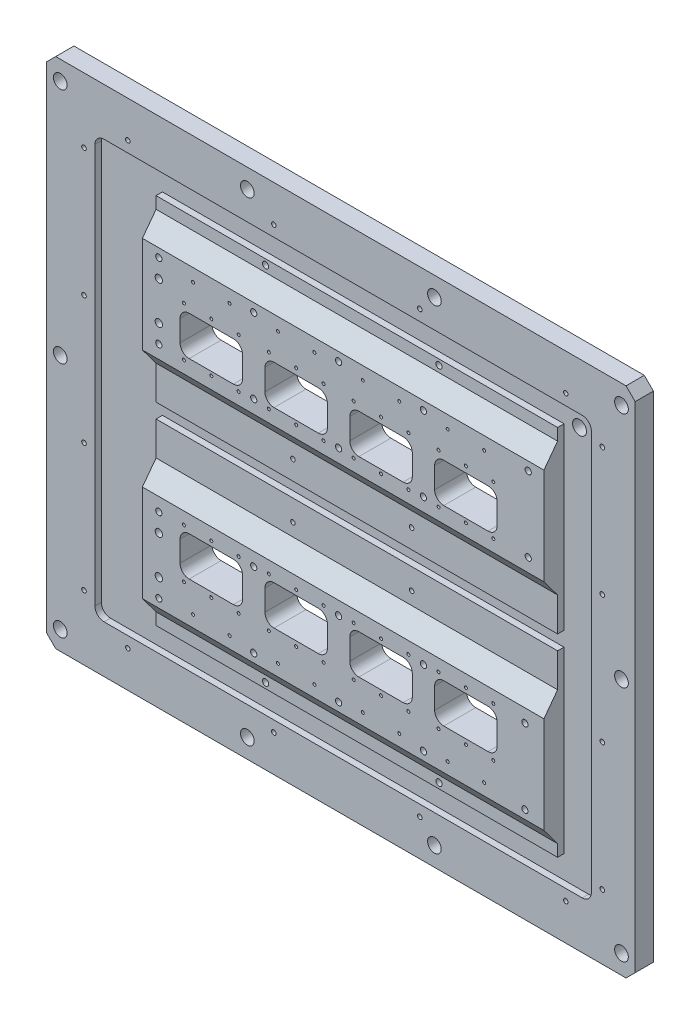
SolidWorks part; units mm, degrees
material "Q235-A"
ref_plane "Front Plane" through (0, 0, 0) normal (0, 0, 1) x (1, 0, 0)
ref_plane "Top Plane" through (0, 0, 0) normal (0, 1, 0) x (1, 0, 0)
ref_plane "Right Plane" through (0, 0, 0) normal (1, 0, 0) x (0, 0, -1)
sketch "Sketch1" plane through (0, 0, 0) normal (0, 0, 1) x (1, 0, 0)
  line L1 (-322.5, -281) -> (322.5, -281)
  line L2 (-322.5, -281) -> (-322.5, 281)
  line L3 (-322.5, 281) -> (322.5, 281)
  line L4 (322.5, -281) -> (322.5, 281)
  line L5 (-322.5, -281) -> (322.5, 281) construction
  line L6 (-322.5, 281) -> (322.5, -281) construction
  point P0 (0, 0)
  dimension "D1" = 562
  dimension "D2" = 645
extrude "Boss-Extrude1" add sketch "Sketch1" along normal blind 20
sketch "Sketch2" plane through (0, 0, 20) normal (0, 0, 1) x (1, 0, 0)
  line L0 (-322.5, 281) -> (-322.5, -281) construction
  line L1 (-269.5, 229) -> (274.5, 229)
  line L2 (-269.5, 229) -> (-269.5, -229)
  line L3 (-269.5, -229) -> (274.5, -229)
  line L4 (274.5, 229) -> (274.5, -229)
  line L5 (-322.5, -281) -> (322.5, -281) construction
  dimension "D1" = 544
  dimension "D2" = 53
  dimension "D3" = 52
  dimension "D4" = 458
extrude "Cut-Extrude1" cut sketch "Sketch2" against normal blind 7
chamfer "Chamfer1" distance 10 angle 45 4 edges at (322.5, -281, 10) (322.5, 281, 10) (-322.5, 281, 10) (-322.5, -281, 10)
ref_plane "Plane1" through (-202.5, 0, 0) normal (1, 0, 0) x (0, 0, -1)
sketch "Sketch3" plane through (-202.5, 0, 0) normal (1, 0, 0) x (0, 0, -1)
  line L0 (-13, 204) -> (-20, 204)
  line L1 (-13, -229) -> (-13, 229) construction
  line L2 (-20, -229) -> (-20, 229) construction
  line L5 (-35, 171) -> (-35, 65)
  line L8 (-20, 8) -> (-13, 8)
  line L9 (-13, 8) -> (-13, 204)
  line L10 (-20, 204) -> (-20, 191)
  line L11 (-20, -8) -> (-20, -45)
  line L14 (-13, -204) -> (-13, -8)
  line L15 (-20, -204) -> (-13, -204)
  line L17 (-13, -8) -> (-20, -8)
  line L18 (-35, -65) -> (-35, -171)
  line L20 (-13, -229) -> (-20, -229) construction
  line L21 (-20, -45) -> (-35, -65)
  line L22 (-20, -204) -> (-20, -191)
  line L23 (-20, -191) -> (-35, -171)
  line L24 (0, -281) -> (-20, -281) construction
  line L25 (0, -271) -> (0, 271) construction
  line L27 (-35, 65) -> (-20, 45)
  line L28 (-20, 45) -> (-20, 8)
  line L29 (-13, 229) -> (-20, 229) construction
  line L30 (-20, 191) -> (-35, 171)
  dimension "D2" = 35
  dimension "D3" = 106
  dimension "D4" = 35
  dimension "D5" = 25
  dimension "D6" = 7
  dimension "D7" = 16
  dimension "D8" = 25
  dimension "D9" = 20
  dimension "D10" = 146
  dimension "D11" = 106
  dimension "D12" = 273
  dimension "D13" = 146
  dimension "D14" = 20
  dimension "D15" = 236
  dimension "D16" = 90
extrude "Boss-Extrude2" add sketch "Sketch3" along normal blind 440
sketch "Sketch4" plane through (0, 0, 35) normal (0, 0, 1) x (1, 0, 0)
  line L0 (-312.5, -281) -> (312.5, -281) construction
  line L1 (-151.25, -83.74) -> (-102.75, -83.74)
  line L2 (-161.25, -93.74) -> (-161.25, -116.74)
  line L3 (-151.25, -126.74) -> (-102.75, -126.74)
  line L4 (-92.75, -93.74) -> (-92.75, -116.74)
  line L5 (-322.5, 271) -> (-322.5, -271) construction
  line L6 (-68.25, -93.74) -> (-68.25, -116.74)
  line L7 (-58.25, -83.74) -> (-9.75, -83.74)
  line L8 (0.25, -93.74) -> (0.25, -116.74)
  line L9 (-58.25, -126.74) -> (-9.75, -126.74)
  line L10 (24.75, -93.74) -> (24.75, -116.74)
  line L11 (34.75, -83.74) -> (83.25, -83.74)
  line L12 (93.25, -93.74) -> (93.25, -116.74)
  line L13 (34.75, -126.74) -> (83.25, -126.74)
  line L14 (117.75, -93.74) -> (117.75, -116.74)
  line L15 (127.75, -83.74) -> (176.25, -83.74)
  line L16 (186.25, -93.74) -> (186.25, -116.74)
  line L17 (127.75, -126.74) -> (176.25, -126.74)
  line L18 (-68.25, 115.5) -> (-68.25, 92.5)
  line L19 (-58.25, 125.5) -> (-9.75, 125.5)
  line L20 (0.25, 115.5) -> (0.25, 92.5)
  line L21 (-58.25, 82.5) -> (-9.75, 82.5)
  line L22 (24.75, 115.5) -> (24.75, 92.5)
  line L23 (34.75, 125.5) -> (83.25, 125.5)
  line L24 (93.25, 115.5) -> (93.25, 92.5)
  line L25 (34.75, 82.5) -> (83.25, 82.5)
  line L26 (117.75, 115.5) -> (117.75, 92.5)
  line L27 (127.75, 125.5) -> (176.25, 125.5)
  line L28 (186.25, 115.5) -> (186.25, 92.5)
  line L29 (127.75, 82.5) -> (176.25, 82.5)
  line L30 (-161.25, 115.5) -> (-161.25, 92.5)
  line L31 (-151.25, 125.5) -> (-102.75, 125.5)
  line L32 (-92.75, 115.5) -> (-92.75, 92.5)
  line L33 (-151.25, 82.5) -> (-102.75, 82.5)
  arc A0 (-102.75, -83.74) -> (-92.75, -93.74) centre (-102.75, -93.74) cw
  arc A1 (-92.75, -116.74) -> (-102.75, -126.74) centre (-102.75, -116.74) cw
  arc A2 (-151.25, -126.74) -> (-161.25, -116.74) centre (-151.25, -116.74) cw
  arc A3 (-161.25, -93.74) -> (-151.25, -83.74) centre (-151.25, -93.74) cw
  arc A4 (-68.25, -93.74) -> (-58.25, -83.74) centre (-58.25, -93.74) cw
  arc A5 (-58.25, -126.74) -> (-68.25, -116.74) centre (-58.25, -116.74) cw
  arc A6 (-9.75, -83.74) -> (0.25, -93.74) centre (-9.75, -93.74) cw
  arc A7 (0.25, -116.74) -> (-9.75, -126.74) centre (-9.75, -116.74) cw
  arc A8 (24.75, -93.74) -> (34.75, -83.74) centre (34.75, -93.74) cw
  arc A9 (34.75, -126.74) -> (24.75, -116.74) centre (34.75, -116.74) cw
  arc A10 (83.25, -83.74) -> (93.25, -93.74) centre (83.25, -93.74) cw
  arc A11 (93.25, -116.74) -> (83.25, -126.74) centre (83.25, -116.74) cw
  arc A12 (117.75, -93.74) -> (127.75, -83.74) centre (127.75, -93.74) cw
  arc A13 (127.75, -126.74) -> (117.75, -116.74) centre (127.75, -116.74) cw
  arc A14 (176.25, -83.74) -> (186.25, -93.74) centre (176.25, -93.74) cw
  arc A15 (186.25, -116.74) -> (176.25, -126.74) centre (176.25, -116.74) cw
  arc A16 (-68.25, 115.5) -> (-58.25, 125.5) centre (-58.25, 115.5) cw
  arc A17 (-58.25, 82.5) -> (-68.25, 92.5) centre (-58.25, 92.5) cw
  arc A18 (-9.75, 125.5) -> (0.25, 115.5) centre (-9.75, 115.5) cw
  arc A19 (0.25, 92.5) -> (-9.75, 82.5) centre (-9.75, 92.5) cw
  arc A20 (24.75, 115.5) -> (34.75, 125.5) centre (34.75, 115.5) cw
  arc A21 (34.75, 82.5) -> (24.75, 92.5) centre (34.75, 92.5) cw
  arc A22 (83.25, 125.5) -> (93.25, 115.5) centre (83.25, 115.5) cw
  arc A23 (93.25, 92.5) -> (83.25, 82.5) centre (83.25, 92.5) cw
  arc A24 (117.75, 115.5) -> (127.75, 125.5) centre (127.75, 115.5) cw
  arc A25 (127.75, 82.5) -> (117.75, 92.5) centre (127.75, 92.5) cw
  arc A26 (176.25, 125.5) -> (186.25, 115.5) centre (176.25, 115.5) cw
  arc A27 (186.25, 92.5) -> (176.25, 82.5) centre (176.25, 92.5) cw
  arc A28 (-161.25, 115.5) -> (-151.25, 125.5) centre (-151.25, 115.5) cw
  arc A29 (-151.25, 82.5) -> (-161.25, 92.5) centre (-151.25, 92.5) cw
  arc A30 (-102.75, 125.5) -> (-92.75, 115.5) centre (-102.75, 115.5) cw
  arc A31 (-92.75, 92.5) -> (-102.75, 82.5) centre (-102.75, 92.5) cw
  point P10 (-92.75, -83.74)
  point P15 (-161.25, -126.74)
  point P18 (-161.25, -83.74)
  dimension "D5" = 10
  dimension "D1" = 68.5
  dimension "D2" = 43
  dimension "D3" = 154.26
  dimension "D4" = 161.25
  dimension "D6" = 4
  dimension "D7" = 2
extrude "Cut-Extrude2" cut sketch "Sketch4" against normal blind 440
sketch "Sketch5" plane through (0, 0, 20) normal (0, 0, 1) x (1, 0, 0)
  line L0 (-312.5, -281) -> (312.5, -281) construction
  line L1 (-322.5, 271) -> (-322.5, -271) construction
  circle A0 centre (-307.5, -260) radius 11.6351
  circle A1 centre (-102.5, -260) radius 11.6351
  circle A2 centre (102.5, -260) radius 11.6351
  circle A3 centre (307.5, -260) radius 11.6351
  circle A4 centre (-102.5, 0) radius 11.6351
  circle A5 centre (102.5, 0) radius 11.6351
  circle A6 centre (307.5, 0) radius 11.6351
  circle A7 centre (-102.5, 260) radius 11.6351
  circle A8 centre (102.5, 260) radius 11.6351
  circle A9 centre (307.5, 260) radius 11.6351
  circle A10 centre (-307.5, 0) radius 11.6351
  circle A11 centre (-307.5, 260) radius 11.6351
  dimension "D1" = 21
  dimension "D2" = 15
  dimension "D3" = 4
  dimension "D4" = 3
hole_wizard "Hole1" positions "Sketch6" profile "Sketch7" legacy end condition through all
sketch "Sketch6" plane through (0, 0, 20) normal (0, 0, 1) x (1, 0, 0)
  point P0 (-307.5, 260)
  point P3 (-102.5, 260)
  point P6 (102.5, 260)
  point P9 (307.5, 260)
  point P12 (307.5, 0)
  point P15 (307.5, -260)
  point P18 (102.5, -260)
  point P21 (-102.5, -260)
  point P24 (-307.5, -260)
  point P27 (-307.5, 0)
sketch "Sketch7" plane through (-307.5, 260, 20) normal (1, 0, 0) x (0, -1, 0)
  line L0 (0, 0) -> (0, 20)
  line L1 (0, 20) -> (4.2, 20)
  line L2 (4.2, 20) -> (4.2, 11)
  line L3 (4.2, 11) -> (7.5, 11)
  line L4 (7.5, 11) -> (7.5, 0)
  line L5 (7.5, 0) -> (0, 0)
  line L6 (0, 110) -> (0, -10) construction
  dimension "直径" = 8.4
  dimension "深度" = 20
  dimension "柱坑直径" = 15
  dimension "柱坑深度" = 11
fillet "Fillet1" radius 10 4 edges at (-269.5, -229, 16.5) (274.5, -229, 16.5) (274.5, 229, 16.5) (-269.5, 229, 16.5)
sketch "Sketch8" plane through (0, 0, 20) normal (0, 0, 1) x (1, 0, 0)
  line L0 (-312.5, -281) -> (312.5, -281) construction
  line L1 (-322.5, 271) -> (-322.5, -271) construction
  circle A0 centre (-281.5, -210) radius 7.3177
  circle A1 centre (286.5, -210) radius 7.3177
  circle A2 centre (286.5, -70) radius 7.3177
  circle A3 centre (286.5, 70) radius 7.3177
  circle A4 centre (286.5, 210) radius 7.3177
  circle A5 centre (-281.5, -70) radius 7.3177
  circle A6 centre (-281.5, 70) radius 7.3177
  circle A7 centre (-281.5, 210) radius 7.3177
  circle A8 centre (-233.5, -241) radius 6.7741
  circle A9 centre (-73.5, -241) radius 6.7741
  circle A10 centre (86.5, -241) radius 6.7741
  circle A11 centre (246.5, -241) radius 6.7741
  circle A12 centre (-73.5, 241) radius 6.7741
  circle A13 centre (86.5, 241) radius 6.7741
  circle A14 centre (246.5, 241) radius 6.7741
  circle A15 centre (-233.5, 241) radius 6.7741
  dimension "D1" = 71
  dimension "D6" = 40
  dimension "D2" = 41
  dimension "D5" = 89
  dimension "D3" = 2
  dimension "D4" = 4
  dimension "D7" = 4
  dimension "D8" = 2
hole_wizard "M6 Tapped Hole1" positions "Sketch9" profile "Sketch10" tap size "M6" standard "GB"
sketch "Sketch9" plane through (0, 0, 20) normal (0, 0, 1) x (1, 0, 0)
  point P0 (-281.5, -210)
  point P3 (-233.5, -241)
  point P6 (-73.5, -241)
  point P9 (86.5, -241)
  point P12 (246.5, -241)
  point P23 (286.5, 70)
  point P26 (286.5, 210)
  point P29 (246.5, 241)
  point P32 (86.5, 241)
  point P35 (-73.5, 241)
  point P38 (-233.5, 241)
  point P41 (-281.5, 210)
  point P44 (-281.5, 70)
  point P50 (286.5, -210)
  point P57 (286.5, -70)
  point P61 (-281.5, -70)
sketch "Sketch10" plane through (-281.5, -210, 20) normal (1, 0, 0) x (0, -1, 0)
  line L0 (0, 0) -> (0, 11.5022)
  line L1 (0, 11.5022) -> (2.5, 10)
  line L2 (2.5, 10) -> (2.5, 0)
  line L5 (2.5, 0) -> (0, 0)
  line L10 (0, 11.5022) -> (-2.5, 10) construction
  line L11 (0, -6.35) -> (0, 107.95) construction
  dimension "螺纹孔钻头直径" = 5
  dimension "螺纹孔钻头深度" = 10
  dimension "导头角度" = 118
cosmetic thread "Cosmetic Thread1" parameters "D1"=10, "D2"=6
cosmetic thread "Cosmetic Thread2" parameters "D1"=10, "D2"=6
cosmetic thread "Cosmetic Thread3" parameters "D1"=10, "D2"=6
cosmetic thread "Cosmetic Thread4" parameters "D1"=10, "D2"=6
cosmetic thread "Cosmetic Thread5" parameters "D1"=10, "D2"=6
cosmetic thread "Cosmetic Thread6" parameters "D1"=10, "D2"=6
cosmetic thread "Cosmetic Thread7" parameters "D1"=10, "D2"=6
cosmetic thread "Cosmetic Thread8" parameters "D1"=10, "D2"=6
cosmetic thread "Cosmetic Thread9" parameters "D1"=10, "D2"=6
cosmetic thread "Cosmetic Thread10" parameters "D1"=10, "D2"=6
cosmetic thread "Cosmetic Thread11" parameters "D1"=10, "D2"=6
cosmetic thread "Cosmetic Thread12" parameters "D1"=10, "D2"=6
cosmetic thread "Cosmetic Thread13" parameters "D1"=10, "D2"=6
cosmetic thread "Cosmetic Thread14" parameters "D1"=10, "D2"=6
cosmetic thread "Cosmetic Thread15" parameters "D1"=10, "D2"=6
cosmetic thread "Cosmetic Thread16" parameters "D1"=10, "D2"=6
sketch "Sketch11" plane through (0, 0, 13) normal (0, 0, 1) x (1, 0, 0)
  line L0 (274.5, -219) -> (274.5, 219) construction
  line L1 (312.5, 281) -> (-312.5, 281) construction
  circle A0 centre (254.5, 209) radius 8.0509
  dimension "D1" = 20
  dimension "D2" = 72
hole_wizard "G3/8 Tapped Hole1" positions "Sketch12" profile "Sketch13" tap size "G3/8" standard "GB" end condition through all
sketch "Sketch12" plane through (0, 0, 13) normal (0, 0, 1) x (1, 0, 0)
  point P0 (254.5, 209)
sketch "Sketch13" plane through (254.5, 209, 13) normal (1, 0, 0) x (0, -1, 0)
  line L0 (0, 0) -> (0, 13)
  line L1 (0, 13) -> (7.625, 13)
  line L2 (7.625, 13) -> (7.625, 0)
  line L5 (7.625, 0) -> (0, 0)
  line L11 (0, -6.35) -> (0, 107.95) construction
  dimension "通孔螺纹孔钻头直径" = 15.25
  dimension "通孔螺纹孔钻头深度" = 13
cosmetic thread "Cosmetic Thread17" parameters "D2"=16.662
sketch "Sketch14" plane through (0, 0, 0) normal (0, 0, -1) x (-1, 0, 0)
  line L0 (312.5, -281) -> (-312.5, -281) construction
  line L1 (322.5, 271) -> (322.5, -271) construction
  circle A0 centre (187.5, -166) radius 10.1136
  circle A1 centre (87.5, -166) radius 10.1136
  circle A2 centre (-12.5, -166) radius 10.1136
  circle A3 centre (-112.5, -166) radius 10.1136
  circle A4 centre (-212.5, -166) radius 10.1136
  circle A5 centre (87.5, -24) radius 10.1136
  circle A6 centre (-12.5, -24) radius 10.1136
  circle A7 centre (-112.5, -24) radius 10.1136
  circle A8 centre (-212.5, -24) radius 10.1136
  circle A9 centre (187.5, -24) radius 10.1136
  circle A10 centre (187.5, 28) radius 10.1136
  circle A11 centre (87.5, 28) radius 10.1136
  circle A12 centre (187.5, 170) radius 10.1136
  circle A13 centre (87.5, 170) radius 10.1136
  circle A14 centre (-12.5, 170) radius 10.1136
  circle A15 centre (-112.5, 170) radius 10.1136
  circle A16 centre (-212.5, 170) radius 10.1136
  circle A17 centre (-212.5, 28) radius 10.1136
  circle A18 centre (-112.5, 28) radius 10.1136
  circle A19 centre (-12.5, 28) radius 10.1136
  dimension "D1" = 115
  dimension "D2" = 135
  dimension "D3" = 5
  dimension "D4" = 2
  dimension "D5" = 2
hole_wizard "M8 Tapped Hole1" positions "Sketch15" profile "Sketch16" tap size "M8" standard "GB"
sketch "Sketch15" plane through (0, 0, 0) normal (0, 0, -1) x (-1, 0, 0)
  point P0 (-212.5, 170)
  point P3 (-112.5, 170)
  point P6 (-12.5, 170)
  point P9 (87.5, 170)
  point P12 (187.5, 170)
  point P15 (187.5, 28)
  point P18 (87.5, 28)
  point P21 (-12.5, 28)
  point P24 (-112.5, 28)
  point P27 (-212.5, 28)
  point P30 (-212.5, -24)
  point P33 (-212.5, -166)
  point P36 (-112.5, -166)
  point P39 (-112.5, -24)
  point P42 (-12.5, -24)
  point P45 (87.5, -24)
  point P48 (187.5, -24)
  point P51 (187.5, -166)
  point P54 (87.5, -166)
  point P57 (-12.5, -166)
sketch "Sketch16" plane through (212.5, 170, 0) normal (1, 0, 0) x (0, 1, 0)
  line L0 (0, 0) -> (0, 18.0429)
  line L1 (0, 18.0429) -> (3.4, 16)
  line L2 (3.4, 16) -> (3.4, 0)
  line L5 (3.4, 0) -> (0, 0)
  line L10 (0, 18.0429) -> (-3.4, 16) construction
  line L11 (0, -6.35) -> (0, 107.95) construction
  dimension "螺纹孔钻头直径" = 6.8
  dimension "螺纹孔钻头深度" = 16
  dimension "导头角度" = 118
cosmetic thread "Cosmetic Thread18" parameters "D1"=16, "D2"=8
cosmetic thread "Cosmetic Thread19" parameters "D1"=16, "D2"=8
cosmetic thread "Cosmetic Thread20" parameters "D1"=16, "D2"=8
cosmetic thread "Cosmetic Thread21" parameters "D1"=16, "D2"=8
cosmetic thread "Cosmetic Thread22" parameters "D1"=16, "D2"=8
cosmetic thread "Cosmetic Thread23" parameters "D1"=16, "D2"=8
cosmetic thread "Cosmetic Thread24" parameters "D1"=16, "D2"=8
cosmetic thread "Cosmetic Thread25" parameters "D1"=16, "D2"=8
cosmetic thread "Cosmetic Thread26" parameters "D1"=16, "D2"=8
cosmetic thread "Cosmetic Thread27" parameters "D1"=16, "D2"=8
cosmetic thread "Cosmetic Thread28" parameters "D1"=16, "D2"=8
cosmetic thread "Cosmetic Thread29" parameters "D1"=16, "D2"=8
cosmetic thread "Cosmetic Thread30" parameters "D1"=16, "D2"=8
cosmetic thread "Cosmetic Thread31" parameters "D1"=16, "D2"=8
cosmetic thread "Cosmetic Thread32" parameters "D1"=16, "D2"=8
cosmetic thread "Cosmetic Thread33" parameters "D1"=16, "D2"=8
cosmetic thread "Cosmetic Thread34" parameters "D1"=16, "D2"=8
cosmetic thread "Cosmetic Thread35" parameters "D1"=16, "D2"=8
cosmetic thread "Cosmetic Thread36" parameters "D1"=16, "D2"=8
cosmetic thread "Cosmetic Thread37" parameters "D1"=16, "D2"=8
sketch "Sketch17" plane through (0, 0, 35) normal (0, 0, 1) x (1, 0, 0)
  line L0 (-322.5, 271) -> (-322.5, -271) construction
  line L1 (-312.5, -281) -> (312.5, -281) construction
  line L4 (-322.5, 0) -> (322.5, 0) construction
  line L5 (322.5, -271) -> (322.5, 271) construction
  line L6 (-184.5, 161.6) -> (-184.5, -161.6) construction
  circle A0 centre (-184.5, -161.6) radius 8.2899
  circle A1 centre (-80.5, -161.6) radius 8.2899
  circle A2 centre (-80.5, -79.6) radius 8.2899
  circle A3 centre (-184.5, -79.6) radius 8.2899
  circle A4 centre (12.5, -161.6) radius 8.2899
  circle A5 centre (12.5, -79.6) radius 8.2899
  circle A6 centre (105.5, -161.6) radius 8.2899
  circle A7 centre (105.5, -79.6) radius 8.2899
  circle A8 centre (216.7, -161.6) radius 8.2899
  circle A9 centre (216.7, -79.6) radius 8.2899
  circle A10 centre (220.3, 79.6) radius 8.2899
  circle A11 centre (220.3, 161.6) radius 8.2899
  circle A12 centre (105.5, 79.6) radius 8.2899
  circle A13 centre (105.5, 161.6) radius 8.2899
  circle A14 centre (12.5, 79.6) radius 8.2899
  circle A15 centre (12.5, 161.6) radius 8.2899
  circle A16 centre (-184.5, 79.6) radius 8.2899
  circle A17 centre (-80.5, 79.6) radius 8.2899
  circle A18 centre (-80.5, 161.6) radius 8.2899
  circle A19 centre (-184.5, 161.6) radius 8.2899
  circle A20 centre (-184.5, 141.6) radius 4.5108
  circle A21 centre (-184.5, 99.6) radius 4.7491
  circle A22 centre (-184.5, -99.6) radius 4.5108
  circle A23 centre (-184.5, -141.6) radius 4.7491
  dimension "D1" = 138
  dimension "D2" = 119.4
  dimension "D8" = 20
  dimension "D9" = 42
  dimension "D10" = 114.8
  dimension "D11" = 114.8
  dimension "D3" = 2
  dimension "D4" = 2
  dimension "D5" = 2
  dimension "D6" = 2
  dimension "D7" = 2
hole_wizard "Hole2" positions "Sketch18" profile "Sketch19" legacy
sketch "Sketch18" plane through (0, 0, 35) normal (0, 0, 1) x (1, 0, 0)
  point P0 (-184.5, 141.6)
  point P3 (-184.5, 99.6)
  point P6 (-184.5, -99.6)
  point P9 (-184.5, -141.6)
sketch "Sketch19" plane through (-184.5, 141.6, 35) normal (1, 0, 0) x (0, -1, 0)
  line L0 (0, 0) -> (0, 8.5)
  line L1 (0, 8.5) -> (4, 8.5)
  line L2 (4, 8.5) -> (4, 0)
  line L3 (4, 0) -> (0, 0)
  line L4 (0, 110) -> (0, -10) construction
  dimension "直径" = 8
  dimension "深度" = 8.5
hole_wizard "M8 Tapped Hole2" positions "Sketch20" profile "Sketch21" tap size "M8" standard "GB"
sketch "Sketch20" plane through (0, 0, 35) normal (0, 0, 1) x (1, 0, 0)
  point P0 (-184.5, 161.6)
  point P3 (-80.5, 161.6)
  point P6 (12.5, 161.6)
  point P9 (105.5, 161.6)
  point P12 (220.3, 161.6)
  point P15 (220.3, 79.6)
  point P18 (105.5, 79.6)
  point P21 (12.5, 79.6)
  point P24 (-80.5, 79.6)
  point P27 (-184.5, 79.6)
  point P30 (-184.5, -79.6)
  point P33 (-184.5, -161.6)
  point P36 (-80.5, -161.6)
  point P39 (-80.5, -79.6)
  point P42 (12.5, -79.6)
  point P45 (12.5, -161.6)
  point P48 (105.5, -161.6)
  point P51 (105.5, -79.6)
  point P54 (216.7, -79.6)
  point P57 (216.7, -161.6)
sketch "Sketch21" plane through (-184.5, 161.6, 35) normal (1, 0, 0) x (0, -1, 0)
  line L0 (0, 0) -> (0, 18.0429)
  line L1 (0, 18.0429) -> (3.4, 16)
  line L2 (3.4, 16) -> (3.4, 0)
  line L5 (3.4, 0) -> (0, 0)
  line L10 (0, 18.0429) -> (-3.4, 16) construction
  line L11 (0, -6.35) -> (0, 107.95) construction
  dimension "螺纹孔钻头直径" = 6.8
  dimension "螺纹孔钻头深度" = 16
  dimension "导头角度" = 118
cosmetic thread "Cosmetic Thread38" parameters "D1"=16, "D2"=8
cosmetic thread "Cosmetic Thread39" parameters "D1"=16, "D2"=8
cosmetic thread "Cosmetic Thread40" parameters "D1"=16, "D2"=8
cosmetic thread "Cosmetic Thread41" parameters "D1"=16, "D2"=8
cosmetic thread "Cosmetic Thread42" parameters "D1"=16, "D2"=8
cosmetic thread "Cosmetic Thread43" parameters "D1"=16, "D2"=8
cosmetic thread "Cosmetic Thread44" parameters "D1"=16, "D2"=8
cosmetic thread "Cosmetic Thread45" parameters "D1"=16, "D2"=8
cosmetic thread "Cosmetic Thread46" parameters "D1"=16, "D2"=8
cosmetic thread "Cosmetic Thread47" parameters "D1"=16, "D2"=8
cosmetic thread "Cosmetic Thread48" parameters "D1"=16, "D2"=8
cosmetic thread "Cosmetic Thread49" parameters "D1"=16, "D2"=8
cosmetic thread "Cosmetic Thread50" parameters "D1"=16, "D2"=8
cosmetic thread "Cosmetic Thread51" parameters "D1"=16, "D2"=8
cosmetic thread "Cosmetic Thread52" parameters "D1"=16, "D2"=8
cosmetic thread "Cosmetic Thread53" parameters "D1"=16, "D2"=8
cosmetic thread "Cosmetic Thread54" parameters "D1"=16, "D2"=8
cosmetic thread "Cosmetic Thread55" parameters "D1"=16, "D2"=8
cosmetic thread "Cosmetic Thread56" parameters "D1"=16, "D2"=8
cosmetic thread "Cosmetic Thread57" parameters "D1"=16, "D2"=8
sketch "Sketch22" plane through (0, 0, 35) normal (0, 0, 1) x (1, 0, 0)
  line L0 (-322.5, 271) -> (-322.5, -271) construction
  line L1 (-312.5, -281) -> (312.5, -281) construction
  circle A0 centre (-147, 157) radius 5.3737
  circle A1 centre (-107, 157) radius 5.3737
  circle A2 centre (-107, -158.24) radius 5.3737
  circle A3 centre (-147, -158.24) radius 5.3737
  circle A4 centre (-54, -158.24) radius 5.3737
  circle A5 centre (-14, -158.24) radius 5.3737
  circle A6 centre (-54, 157) radius 5.3737
  circle A7 centre (-14, 157) radius 5.3737
  circle A8 centre (39, -158.24) radius 5.3737
  circle A9 centre (79, -158.24) radius 5.3737
  circle A10 centre (39, 157) radius 5.3737
  circle A11 centre (79, 157) radius 5.3737
  circle A12 centre (132, -158.24) radius 5.3737
  circle A13 centre (172, -158.24) radius 5.3737
  circle A14 centre (132, 157) radius 5.3737
  circle A15 centre (172, 157) radius 5.3737
  dimension "D2" = 438
  dimension "D1" = 175.5
  dimension "D3" = 2
  dimension "D4" = 2
  dimension "D5" = 4
hole_wizard "M4 Tapped Hole1" positions "Sketch23" profile "Sketch24" tap size "M4" standard "GB"
sketch "Sketch23" plane through (0, 0, 35) normal (0, 0, 1) x (1, 0, 0)
  point P0 (-147, 157)
  point P3 (-107, 157)
  point P6 (-54, 157)
  point P9 (-14, 157)
  point P12 (39, 157)
  point P15 (79, 157)
  point P18 (132, 157)
  point P21 (172, 157)
  point P24 (-147, -158.24)
  point P27 (-107, -158.24)
  point P30 (-54, -158.24)
  point P33 (-14, -158.24)
  point P36 (39, -158.24)
  point P39 (79, -158.24)
  point P42 (132, -158.24)
  point P45 (172, -158.24)
sketch "Sketch24" plane through (-147, 157, 35) normal (1, 0, 0) x (0, -1, 0)
  line L0 (0, 0) -> (0, 8.9914)
  line L1 (0, 8.9914) -> (1.65, 8)
  line L2 (1.65, 8) -> (1.65, 0)
  line L5 (1.65, 0) -> (0, 0)
  line L10 (0, 8.9914) -> (-1.65, 8) construction
  line L11 (0, -6.35) -> (0, 107.95) construction
  dimension "螺纹孔钻头直径" = 3.3
  dimension "螺纹孔钻头深度" = 8
  dimension "导头角度" = 118
cosmetic thread "Cosmetic Thread58" parameters "D1"=8, "D2"=4
cosmetic thread "Cosmetic Thread59" parameters "D1"=8, "D2"=4
cosmetic thread "Cosmetic Thread60" parameters "D1"=8, "D2"=4
cosmetic thread "Cosmetic Thread61" parameters "D1"=8, "D2"=4
cosmetic thread "Cosmetic Thread62" parameters "D1"=8, "D2"=4
cosmetic thread "Cosmetic Thread63" parameters "D1"=8, "D2"=4
cosmetic thread "Cosmetic Thread64" parameters "D1"=8, "D2"=4
cosmetic thread "Cosmetic Thread65" parameters "D1"=8, "D2"=4
cosmetic thread "Cosmetic Thread66" parameters "D1"=8, "D2"=4
cosmetic thread "Cosmetic Thread67" parameters "D1"=8, "D2"=4
cosmetic thread "Cosmetic Thread68" parameters "D1"=8, "D2"=4
cosmetic thread "Cosmetic Thread69" parameters "D1"=8, "D2"=4
cosmetic thread "Cosmetic Thread70" parameters "D1"=8, "D2"=4
cosmetic thread "Cosmetic Thread71" parameters "D1"=8, "D2"=4
cosmetic thread "Cosmetic Thread72" parameters "D1"=8, "D2"=4
cosmetic thread "Cosmetic Thread73" parameters "D1"=8, "D2"=4
sketch "Sketch25" plane through (0, 0, 35) normal (0, 0, 1) x (1, 0, 0)
  line L0 (-151.25, -126.74) -> (-102.75, -126.74) construction
  line L1 (-161.25, -93.74) -> (-161.25, -116.74) construction
  line L2 (-269.5, 0) -> (274.5, 0) construction
  line L3 (-269.5, 219) -> (-269.5, -219) construction
  line L4 (274.5, -219) -> (274.5, 219) construction
  circle A0 centre (-157, -132.24) radius 4.0006
  circle A1 centre (-157, -78.24) radius 4.0006
  circle A2 centre (-127, -78.24) radius 4.0006
  circle A3 centre (-97, -78.24) radius 4.0006
  circle A4 centre (-127, -132.24) radius 4.0006
  circle A5 centre (-97, -132.24) radius 4.0006
  circle A6 centre (-64, -132.24) radius 4.0006
  circle A7 centre (-64, -78.24) radius 4.0006
  circle A8 centre (-34, -78.24) radius 4.0006
  circle A9 centre (-4, -78.24) radius 4.0006
  circle A10 centre (-34, -132.24) radius 4.0006
  circle A11 centre (-4, -132.24) radius 4.0006
  circle A12 centre (29, -132.24) radius 4.0006
  circle A13 centre (29, -78.24) radius 4.0006
  circle A14 centre (59, -78.24) radius 4.0006
  circle A15 centre (89, -78.24) radius 4.0006
  circle A16 centre (59, -132.24) radius 4.0006
  circle A17 centre (89, -132.24) radius 4.0006
  circle A18 centre (122, -132.24) radius 4.0006
  circle A19 centre (122, -78.24) radius 4.0006
  circle A20 centre (152, -78.24) radius 4.0006
  circle A21 centre (182, -78.24) radius 4.0006
  circle A22 centre (152, -132.24) radius 4.0006
  circle A23 centre (182, -132.24) radius 4.0006
  circle A24 centre (182, 132.24) radius 4.0006
  circle A25 centre (152, 132.24) radius 4.0006
  circle A26 centre (182, 78.24) radius 4.0006
  circle A27 centre (152, 78.24) radius 4.0006
  circle A28 centre (122, 78.24) radius 4.0006
  circle A29 centre (122, 132.24) radius 4.0006
  circle A30 centre (89, 132.24) radius 4.0006
  circle A31 centre (59, 132.24) radius 4.0006
  circle A32 centre (89, 78.24) radius 4.0006
  circle A33 centre (59, 78.24) radius 4.0006
  circle A34 centre (29, 78.24) radius 4.0006
  circle A35 centre (29, 132.24) radius 4.0006
  circle A36 centre (-4, 132.24) radius 4.0006
  circle A37 centre (-34, 132.24) radius 4.0006
  circle A38 centre (-4, 78.24) radius 4.0006
  circle A39 centre (-34, 78.24) radius 4.0006
  circle A40 centre (-64, 78.24) radius 4.0006
  circle A41 centre (-64, 132.24) radius 4.0006
  circle A42 centre (-97, 132.24) radius 4.0006
  circle A43 centre (-127, 132.24) radius 4.0006
  circle A44 centre (-97, 78.24) radius 4.0006
  circle A45 centre (-127, 78.24) radius 4.0006
  circle A46 centre (-157, 78.24) radius 4.0006
  circle A47 centre (-157, 132.24) radius 4.0006
  dimension "D2" = 4.25
  dimension "D1" = 5.5
  dimension "D3" = 2
  dimension "D4" = 3
  dimension "D5" = 4
hole_wizard "M4 Tapped Hole2" positions "Sketch26" profile "Sketch27" tap size "M4" standard "GB"
sketch "Sketch26" plane through (0, 0, 35) normal (0, 0, 1) x (1, 0, 0)
  point P0 (-157, -78.24)
  point P3 (-127, -78.24)
  point P6 (-97, -78.24)
  point P9 (-157, -132.24)
  point P12 (-127, -132.24)
  point P15 (-97, -132.24)
  point P18 (-64, -78.24)
  point P21 (-34, -78.24)
  point P24 (-4, -78.24)
  point P29 (-34, -132.24)
  point P32 (-64, -132.24)
  point P35 (-4, -132.24)
  point P38 (29, -78.24)
  point P41 (59, -78.24)
  point P44 (89, -78.24)
  point P47 (122, -78.24)
  point P50 (122, -132.24)
  point P53 (89, -132.24)
  point P56 (59, -132.24)
  point P59 (29, -132.24)
  point P62 (152, -78.24)
  point P65 (182, -78.24)
  point P68 (182, -132.24)
  point P71 (152, -132.24)
  point P75 (-157, 132.24)
  point P78 (-157, 78.24)
  point P81 (-127, 78.24)
  point P84 (-97, 78.24)
  point P87 (-97, 132.24)
  point P90 (-127, 132.24)
  point P93 (-64, 132.24)
  point P96 (-34, 132.24)
  point P99 (-4, 132.24)
  point P102 (29, 132.24)
  point P105 (59, 132.24)
  point P108 (89, 132.24)
  point P111 (89, 78.24)
  point P114 (59, 78.24)
  point P117 (29, 78.24)
  point P120 (-4, 78.24)
  point P123 (-34, 78.24)
  point P126 (-64, 78.24)
  point P129 (122, 132.24)
  point P134 (122, 78.24)
  point P137 (152, 78.24)
  point P140 (182, 78.24)
  point P147 (152, 132.24)
  point P150 (182, 132.24)
sketch "Sketch27" plane through (-157, -78.24, 35) normal (1, 0, 0) x (0, -1, 0)
  line L0 (0, 0) -> (0, 8.9914)
  line L1 (0, 8.9914) -> (1.65, 8)
  line L2 (1.65, 8) -> (1.65, 0)
  line L5 (1.65, 0) -> (0, 0)
  line L10 (0, 8.9914) -> (-1.65, 8) construction
  line L11 (0, -6.35) -> (0, 107.95) construction
  dimension "螺纹孔钻头直径" = 3.3
  dimension "螺纹孔钻头深度" = 8
  dimension "导头角度" = 118
cosmetic thread "Cosmetic Thread74" parameters "D1"=8, "D2"=4
cosmetic thread "Cosmetic Thread75" parameters "D1"=8, "D2"=4
cosmetic thread "Cosmetic Thread76" parameters "D1"=8, "D2"=4
cosmetic thread "Cosmetic Thread77" parameters "D1"=8, "D2"=4
cosmetic thread "Cosmetic Thread78" parameters "D1"=8, "D2"=4
cosmetic thread "Cosmetic Thread79" parameters "D1"=8, "D2"=4
cosmetic thread "Cosmetic Thread80" parameters "D1"=8, "D2"=4
cosmetic thread "Cosmetic Thread81" parameters "D1"=8, "D2"=4
cosmetic thread "Cosmetic Thread82" parameters "D1"=8, "D2"=4
cosmetic thread "Cosmetic Thread83" parameters "D1"=8, "D2"=4
cosmetic thread "Cosmetic Thread84" parameters "D1"=8, "D2"=4
cosmetic thread "Cosmetic Thread85" parameters "D1"=8, "D2"=4
cosmetic thread "Cosmetic Thread86" parameters "D1"=8, "D2"=4
cosmetic thread "Cosmetic Thread87" parameters "D1"=8, "D2"=4
cosmetic thread "Cosmetic Thread88" parameters "D1"=8, "D2"=4
cosmetic thread "Cosmetic Thread89" parameters "D1"=8, "D2"=4
cosmetic thread "Cosmetic Thread90" parameters "D1"=8, "D2"=4
cosmetic thread "Cosmetic Thread91" parameters "D1"=8, "D2"=4
cosmetic thread "Cosmetic Thread92" parameters "D1"=8, "D2"=4
cosmetic thread "Cosmetic Thread93" parameters "D1"=8, "D2"=4
cosmetic thread "Cosmetic Thread94" parameters "D1"=8, "D2"=4
cosmetic thread "Cosmetic Thread95" parameters "D1"=8, "D2"=4
cosmetic thread "Cosmetic Thread96" parameters "D1"=8, "D2"=4
cosmetic thread "Cosmetic Thread97" parameters "D1"=8, "D2"=4
cosmetic thread "Cosmetic Thread98" parameters "D1"=8, "D2"=4
cosmetic thread "Cosmetic Thread99" parameters "D1"=8, "D2"=4
cosmetic thread "Cosmetic Thread100" parameters "D1"=8, "D2"=4
cosmetic thread "Cosmetic Thread101" parameters "D1"=8, "D2"=4
cosmetic thread "Cosmetic Thread102" parameters "D1"=8, "D2"=4
cosmetic thread "Cosmetic Thread103" parameters "D1"=8, "D2"=4
cosmetic thread "Cosmetic Thread104" parameters "D1"=8, "D2"=4
cosmetic thread "Cosmetic Thread105" parameters "D1"=8, "D2"=4
cosmetic thread "Cosmetic Thread106" parameters "D1"=8, "D2"=4
cosmetic thread "Cosmetic Thread107" parameters "D1"=8, "D2"=4
cosmetic thread "Cosmetic Thread108" parameters "D1"=8, "D2"=4
cosmetic thread "Cosmetic Thread109" parameters "D1"=8, "D2"=4
cosmetic thread "Cosmetic Thread110" parameters "D1"=8, "D2"=4
cosmetic thread "Cosmetic Thread111" parameters "D1"=8, "D2"=4
cosmetic thread "Cosmetic Thread112" parameters "D1"=8, "D2"=4
cosmetic thread "Cosmetic Thread113" parameters "D1"=8, "D2"=4
cosmetic thread "Cosmetic Thread114" parameters "D1"=8, "D2"=4
cosmetic thread "Cosmetic Thread115" parameters "D1"=8, "D2"=4
cosmetic thread "Cosmetic Thread116" parameters "D1"=8, "D2"=4
cosmetic thread "Cosmetic Thread117" parameters "D1"=8, "D2"=4
cosmetic thread "Cosmetic Thread118" parameters "D1"=8, "D2"=4
cosmetic thread "Cosmetic Thread119" parameters "D1"=8, "D2"=4
cosmetic thread "Cosmetic Thread120" parameters "D1"=8, "D2"=4
cosmetic thread "Cosmetic Thread121" parameters "D1"=8, "D2"=4
sketch "Sketch28" plane through (0, 0, 20) normal (0, 0, 1) x (1, 0, 0)
  line L0 (-322.5, 271) -> (-322.5, -271) construction
  line L1 (-52.5, 29) -> (77.5, 29)
  line L2 (-52.5, 29) -> (-52.5, -31)
  line L3 (-52.5, -31) -> (77.5, -31)
  line L4 (77.5, 29) -> (77.5, -31)
  line L5 (-312.5, -281) -> (312.5, -281) construction
  line L6 (312.5, 281) -> (-312.5, 281) construction
  line L7 (-82.5, 198) -> (107.5, 198)
  line L8 (-82.5, 198) -> (-82.5, -198)
  line L9 (-82.5, -198) -> (107.5, -198)
  line L10 (107.5, 198) -> (107.5, -198)
  dimension "D1" = 130
  dimension "D2" = 60
  dimension "D3" = 270
  dimension "D4" = 250
  dimension "D5" = 190
  dimension "D6" = 240
  dimension "D7" = 396
  dimension "D8" = 83
hole_wizard "M6 Tapped Hole2" positions "Sketch29" profile "Sketch30" tap size "M6" standard "GB"
sketch "Sketch29" plane through (0, 0, 20) normal (0, 0, 1) x (1, 0, 0)
  point P0 (-52.5, 29)
  point P3 (-52.5, -31)
  point P6 (77.5, -31)
  point P9 (77.5, 29)
sketch "Sketch30" plane through (-52.5, 29, 20) normal (1, 0, 0) x (0, -1, 0)
  line L0 (0, 0) -> (0, 13.5022)
  line L1 (0, 13.5022) -> (2.5, 12)
  line L2 (2.5, 12) -> (2.5, 0)
  line L5 (2.5, 0) -> (0, 0)
  line L10 (0, 13.5022) -> (-2.5, 12) construction
  line L11 (0, -6.35) -> (0, 107.95) construction
  dimension "螺纹孔钻头直径" = 5
  dimension "螺纹孔钻头深度" = 12
  dimension "导头角度" = 118
cosmetic thread "Cosmetic Thread122" parameters "D1"=12, "D2"=6
cosmetic thread "Cosmetic Thread123" parameters "D1"=12, "D2"=6
cosmetic thread "Cosmetic Thread124" parameters "D1"=12, "D2"=6
cosmetic thread "Cosmetic Thread125" parameters "D1"=12, "D2"=6
hole_wizard "M8 Tapped Hole3" positions "Sketch31" profile "Sketch32" tap size "M8" standard "GB"
sketch "Sketch31" plane through (0, 0, 20) normal (0, 0, 1) x (1, 0, 0)
  point P0 (-82.5, -198)
  point P3 (107.5, -198)
  point P6 (-82.5, 198)
  point P9 (107.5, 198)
sketch "Sketch32" plane through (-82.5, -198, 20) normal (1, 0, 0) x (0, -1, 0)
  line L0 (0, 0) -> (0, 18.0429)
  line L1 (0, 18.0429) -> (3.4, 16)
  line L2 (3.4, 16) -> (3.4, 0)
  line L5 (3.4, 0) -> (0, 0)
  line L10 (0, 18.0429) -> (-3.4, 16) construction
  line L11 (0, -6.35) -> (0, 107.95) construction
  dimension "螺纹孔钻头直径" = 6.8
  dimension "螺纹孔钻头深度" = 16
  dimension "导头角度" = 118
cosmetic thread "Cosmetic Thread126" parameters "D1"=16, "D2"=8
cosmetic thread "Cosmetic Thread127" parameters "D1"=16, "D2"=8
cosmetic thread "Cosmetic Thread128" parameters "D1"=16, "D2"=8
cosmetic thread "Cosmetic Thread129" parameters "D1"=16, "D2"=8
